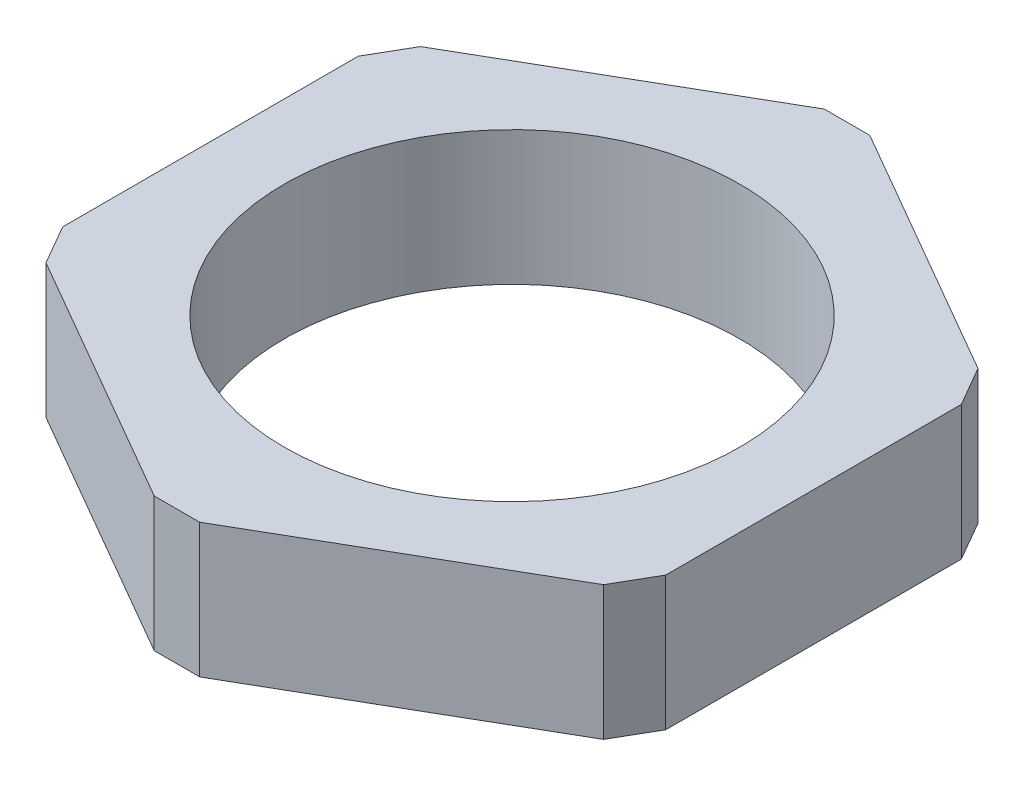
from build123d import *

# Parameters (mm, degrees)
BOSS_EXTRUDE1_DEPTH        = 10
M36X2_0_TAPPED_HOLE1_D     = 34
M36X2_0_TAPPED_HOLE1_DEPTH = 82
M36X2_0_TAPPED_HOLE1_TIP   = 10.214630523
SKETCH4_W                  = 19.309531336
SKETCH4_H                  = 7.869851007
CUT_EXTRUDE1_DEPTH         = 88
CIRPATTERN1_COUNT          = 6


with BuildPart() as part:
    # Sketch1 → Boss-Extrude1 (new body)
    with BuildSketch(Plane(origin=(0, 0, 0), x_dir=(1, 0, 0), z_dir=(0, 1, 0))):
        Polygon((22.5, -12.990381057), (22.5, 12.990381057), (0, 25.980762114), (-22.5, 12.990381057), (-22.5, -12.990381057), (0, -25.980762114), align=None)
    extrude(amount=BOSS_EXTRUDE1_DEPTH)

    # M36x2.0 Tapped Hole1
    with Locations(Plane(origin=(0, 10, 0), x_dir=(1, 0, 0), z_dir=(0, 1, 0))):
        with Locations((0, 0)):
            Hole(M36X2_0_TAPPED_HOLE1_D / 2, depth=M36X2_0_TAPPED_HOLE1_DEPTH)
            with Locations((0, 0, -(M36X2_0_TAPPED_HOLE1_DEPTH + M36X2_0_TAPPED_HOLE1_TIP / 2))):  # 118° drill point
                Cone(0, M36X2_0_TAPPED_HOLE1_D / 2, M36X2_0_TAPPED_HOLE1_TIP, mode=Mode.SUBTRACT)

    # Sketch4 → Cut-Extrude1 (cut)
    with BuildSketch(Plane(origin=(0, 10, 0), x_dir=(1, 0, 0), z_dir=(0, 1, 0))):
        with Locations((1.413316262, 28.934925504)):
            Rectangle(SKETCH4_W, SKETCH4_H)
    cut_extrude1 = extrude(amount=-CUT_EXTRUDE1_DEPTH, mode=Mode.SUBTRACT)

    # CirPattern1: Cut-Extrude1 ×6 about axis
    cirpattern1_axis = Axis((0, 0, 0), (0, 1, 0))
    for i in range(1, CIRPATTERN1_COUNT):
        add(cut_extrude1.rotate(cirpattern1_axis, i * 360 / CIRPATTERN1_COUNT), mode=Mode.SUBTRACT)


solid = part.part
